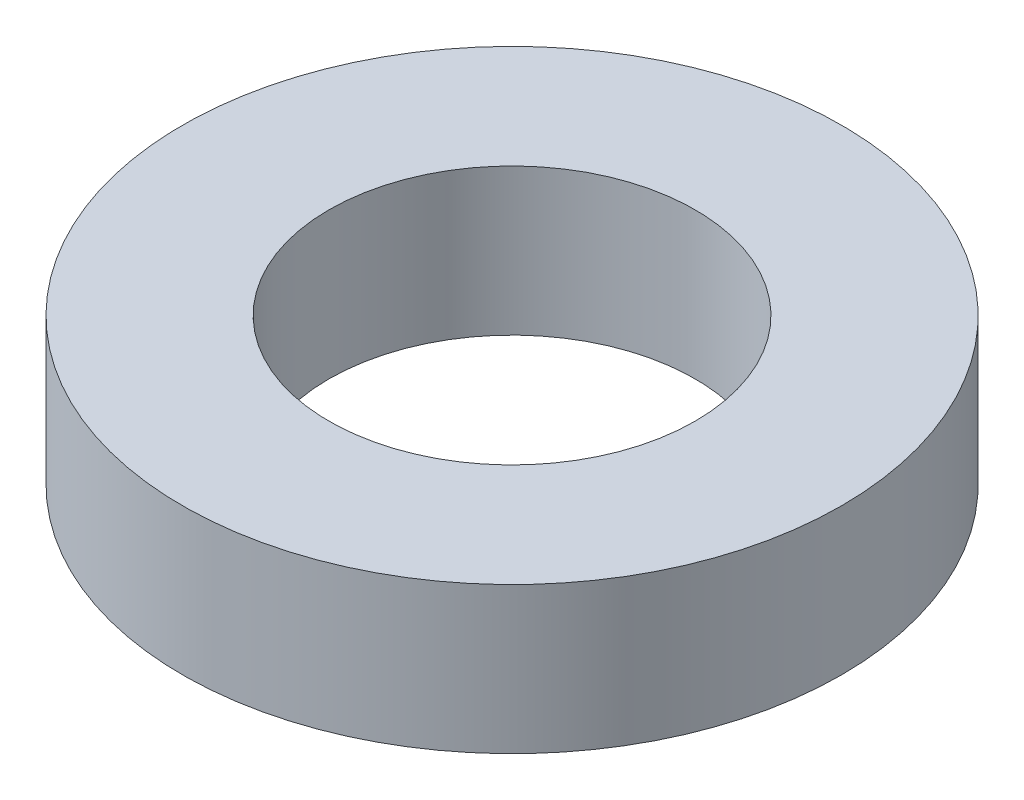
SolidWorks part; units mm, degrees
material "Plain Carbon Steel"
ref_plane "Front Plane" through (0, 0, 0) normal (0, 0, 1) x (1, 0, 0)
ref_plane "Top Plane" through (0, 0, 0) normal (0, 1, 0) x (1, 0, 0)
ref_plane "Right Plane" through (0, 0, 0) normal (1, 0, 0) x (0, 0, -1)
sketch "Sketch1" plane through (0, 0, 0) normal (0, 0, 1) x (1, 0, 0)
  line L0 (0, -473.3811) -> (0, 23195.6752) construction
  line L2 (5, 0) -> (9, 0)
  line L3 (5, 0) -> (5, -4)
  line L4 (5, -4) -> (9, -4)
  line L5 (9, 0) -> (9, -4)
  dimension "D1" = 4
  dimension "D2" = 5
  dimension "D3" = 9
revolve "Revolve1" add sketch "Sketch1" angle 360 about L0
